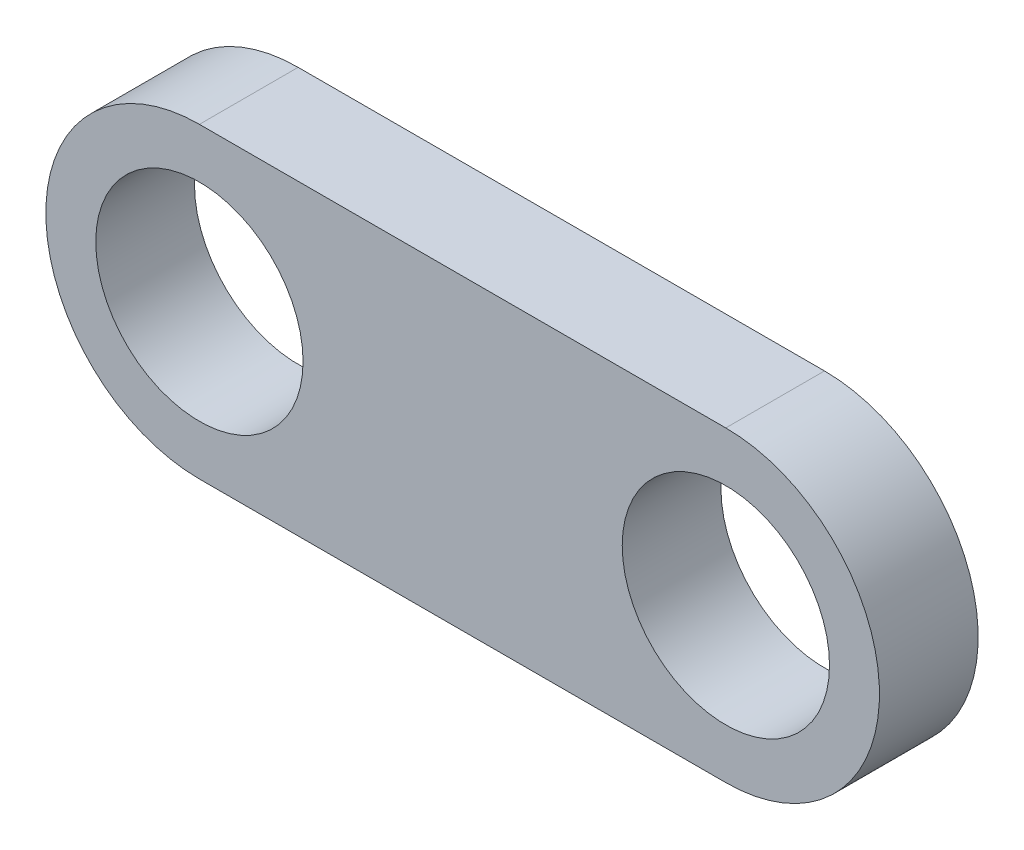
from build123d import *

# Parameters (mm, degrees)
SKETCH1_R           = 3.674588618
BOSS_EXTRUDE1_DEPTH = 3.5


with BuildPart() as part:
    # Sketch1 → Boss-Extrude1 (new body)
    with BuildSketch(Plane.XY):
        with BuildLine():
            Line((26.125402815, 5.46233555), (7.464079644, 5.452693539))
            ThreePointArc((7.464079644, 5.452693539), (2.01909867, 0.007712565), (7.464079644, -5.43726841))
            Line((7.464079644, -5.43726841), (7.46970589, -5.437265503))
            Line((7.46970589, -5.437265503), (26.128216151, -5.427625672))
            ThreePointArc((26.128216151, -5.427625672), (31.573196944, 0.01876197), (26.125402815, 5.46233555))
        make_face()
        with Locations((7.464079644, 0.007712565)):
            Circle(SKETCH1_R, mode=Mode.SUBTRACT)
        with Locations((26.128216151, 0.017355302)):
            Circle(SKETCH1_R, mode=Mode.SUBTRACT)
    extrude(amount=BOSS_EXTRUDE1_DEPTH)


solid = part.part
